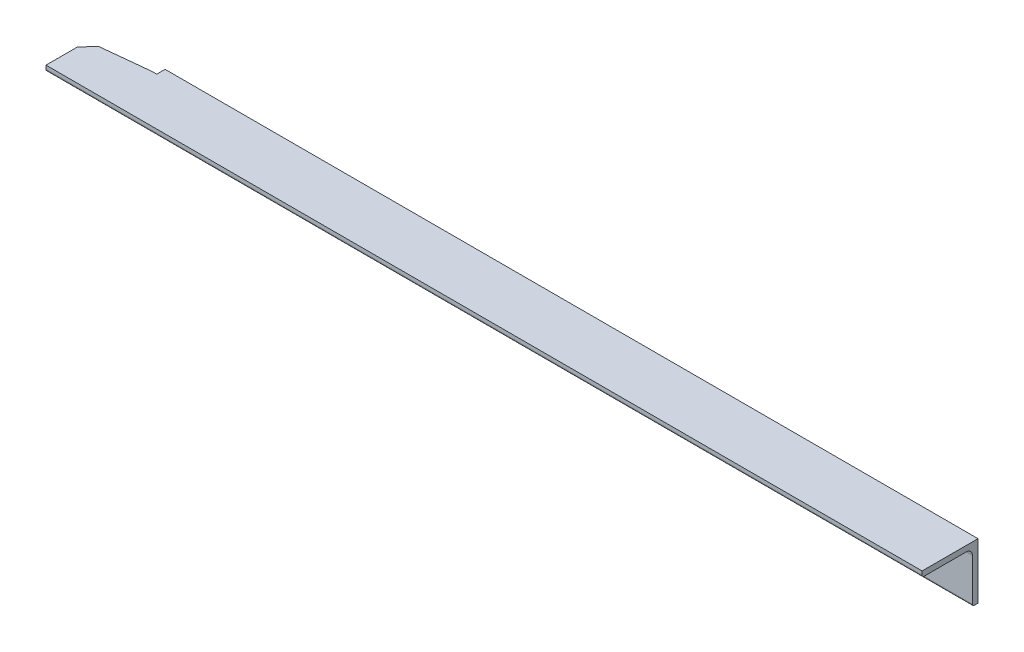
SolidWorks part; units mm, degrees
material "SPCC冷轧板喷塑"
ref_plane "前视基准面" through (0, 0, 0) normal (0, 0, 1) x (1, 0, 0)
ref_plane "上视基准面" through (0, 0, 0) normal (0, 1, 0) x (1, 0, 0)
ref_plane "右视基准面" through (0, 0, 0) normal (1, 0, 0) x (0, 0, -1)
other "Configuration Table"
sketch "草图1" plane through (0, 0, 0) normal (0, 0, 1) x (1, 0, 0)
  line L0 (391.75, 0) -> (-391.75, 0)
  point P4 (0, 0)
  dimension "D1" = 783.5
other "Gbt706-2008 热轧等边角钢 050×5(1)"
ref_plane "基准面1" through (391.75, 0, 0) normal (-1, 0, 0) x (0, -1, 0)
sketch "Sketch1" plane through (391.75, 0, 0) normal (-1, 0, 0) x (0, -1, 0)
  line L0 (0, 0) -> (0, 50)
  line L1 (0, 25) -> (5, 25) construction
  line L2 (5, 48.3333) -> (5, 10.5)
  line L3 (10.5, 5) -> (48.3333, 5)
  line L4 (25, 5) -> (25, 0) construction
  line L5 (50, 0) -> (0, 0)
  line L6 (0, 50) -> (3.3333, 50)
  line L7 (50, 0) -> (50, 3.3333)
  arc A0 (50, 3.3333) -> (48.3333, 5) centre (48.3333, 3.3333) ccw
  arc A1 (3.3333, 50) -> (5, 48.3333) centre (3.3333, 48.3333) cw
  arc A2 (10.5, 5) -> (5, 10.5) centre (10.5, 10.5) cw
  point P10 (25, 0)
  point P14 (0, 25)
  point P15 (5, 25)
  point P16 (25, 5)
  point P17 (5, 50)
  point P18 (50, 5)
  point P21 (50, 5)
  point P24 (5, 50)
  point P25 (0, 0)
sketch "草图2" plane through (0, 0, 0) normal (0, 1, 0) x (1, 0, 0)
  line L0 (-335.25, 0) -> (-335.25, -7.5014)
  line L1 (-391.75, 0) -> (391.75, 0) construction
  line L2 (-335.25, -2.5288) -> (-335.25, 0) construction
  line L3 (-339.7274, -7.5014) -> (-382.7953, -12.028)
  line L4 (-382.7953, -12.028) -> (-391.75, -21.9732)
  line L5 (-391.75, -50) -> (-391.75, 0) construction
  line L6 (-391.75, -21.9732) -> (-382.7953, -12.028) construction
  line L7 (-391.75, -21.9732) -> (-391.75, -52.5014)
  line L8 (-391.75, -138.0268) -> (-391.75, -21.9732) construction
  line L9 (-391.75, -52.5014) -> (-406.75, -52.5014)
  line L10 (-406.75, -52.5014) -> (-406.75, 7.4986)
  line L11 (-406.75, 7.4986) -> (-335.25, 7.4986)
  line L12 (-335.25, 7.4986) -> (-335.25, 0)
  line L13 (-335.25, -7.5014) -> (-339.7274, -7.5014)
  dimension "D1" = 15
  dimension "D2" = 15
  dimension "D3" = 60
extrude "切除-拉伸1" cut sketch "草图2" against normal through all
equation "\"D2@Sketch1\"= \"D1@Sketch1\" / 3"
